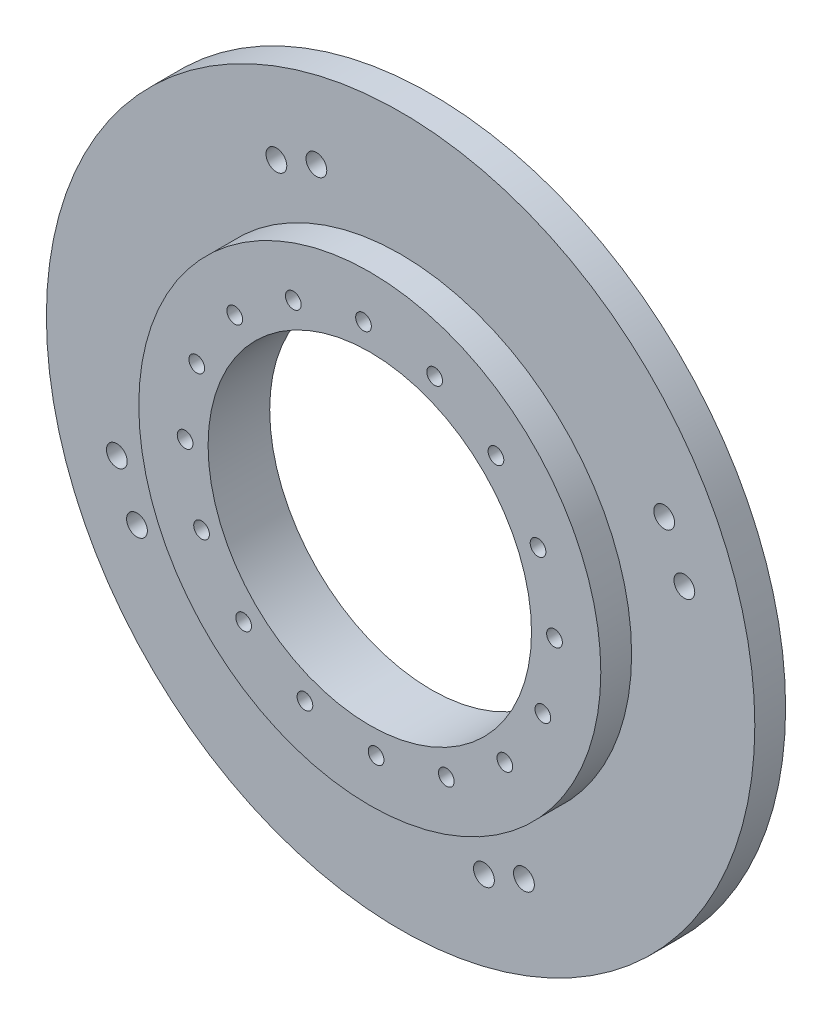
SolidWorks part; units mm, degrees
ref_plane "前视基准面" through (0, 0, 0) normal (0, 0, 1) x (1, 0, 0)
ref_plane "上视基准面" through (0, 0, 0) normal (0, 1, 0) x (1, 0, 0)
ref_plane "右视基准面" through (0, 0, 0) normal (1, 0, 0) x (0, 0, -1)
sketch "草图1" plane through (0, 0, 0) normal (0, 0, 1) x (1, 0, 0)
  circle A0 centre (0, 0) radius 230
  dimension "D1" = 460
extrude "凸台-拉伸1" add sketch "草图1" along normal mid plane 20
sketch "草图2" plane through (0, 0, -10) normal (0, 0, -1) x (-1, 0, 0)
  circle A0 centre (0, 0) radius 105
  dimension "D1" = 210
extrude "切除-拉伸1" cut sketch "草图2" against normal through all
sketch "草图3" plane through (0, 0, 10) normal (0, 0, 1) x (1, 0, 0)
  circle A0 centre (0, 0) radius 105
  circle A1 centre (0, 0) radius 150
  dimension "D1" = 210
  dimension "D2" = 300
extrude "凸台-拉伸2" add sketch "草图3" along normal blind 20
hole_wizard "M12 螺纹孔1" positions "草图5" profile "草图4" tap size "M12" standard "GB" end condition through all
sketch "草图5" plane through (0, 0, 30) normal (0, 0, 1) x (1, 0, 0)
  circle A0 centre (112.3657, -42.1183) radius 7 construction
  point P1 (112.3657, -42.1183)
cosmetic thread "孔螺蚊线1" parameters "D2"=12
sketch "草图4" plane through (112.3657, -42.1183, 30) normal (1, 0, 0) x (0, -1, 0)
  line L0 (0, 0) -> (0, 40)
  line L1 (0, 40) -> (5.1, 40)
  line L2 (5.1, 40) -> (5.1, 0)
  line L5 (5.1, 0) -> (0, 0)
  line L11 (0, -6.35) -> (0, 107.95) construction
  dimension "通孔螺纹孔钻头直径" = 10.2
  dimension "通孔螺纹孔钻头深度" = 40
pattern_circular "阵列(圆周)1" count 16 over 360 about axis through (0, 0, 0) along (0, 0, 1) of "M12 螺纹孔1"
hole_wizard "M12 间隙孔1" positions "草图7" profile "草图6" hole size "M12" standard "GB"
sketch "草图7" plane through (0, 0, 10) normal (0, 0, 1) x (1, 0, 0)
  circle A0 centre (54.1187, -171.7192) radius 5 construction
  circle A1 centre (80.0886, -161.2518) radius 5 construction
  circle A2 centre (171.1659, 87.8581) radius 5 construction
  circle A3 centre (184.2501, 55.3958) radius 5 construction
  circle A4 centre (-171.1659, -87.8581) radius 5 construction
  circle A5 centre (-184.2501, -55.3958) radius 5 construction
  circle A6 centre (-80.6492, 162.6427) radius 5 construction
  circle A7 centre (-54.6793, 173.1101) radius 5 construction
  point P1 (54.1187, -171.7192)
  point P4 (80.0886, -161.2518)
  point P7 (171.1659, 87.8581)
  point P10 (184.2501, 55.3958)
  point P13 (-171.1659, -87.8581)
  point P16 (-184.2501, -55.3958)
  point P19 (-80.6492, 162.6427)
  point P22 (-54.6793, 173.1101)
sketch "草图6" plane through (54.1187, -171.7192, 10) normal (1, 0, 0) x (0, -1, 0)
  line L0 (0, 0) -> (0, 20)
  line L1 (0, 20) -> (6.75, 20)
  line L2 (6.75, 20) -> (6.75, 0)
  line L5 (6.75, 0) -> (0, 0)
  line L11 (0, -6.35) -> (0, 107.95) construction
  dimension "通孔孔直径" = 13.5
  dimension "通孔孔深度" = 20
